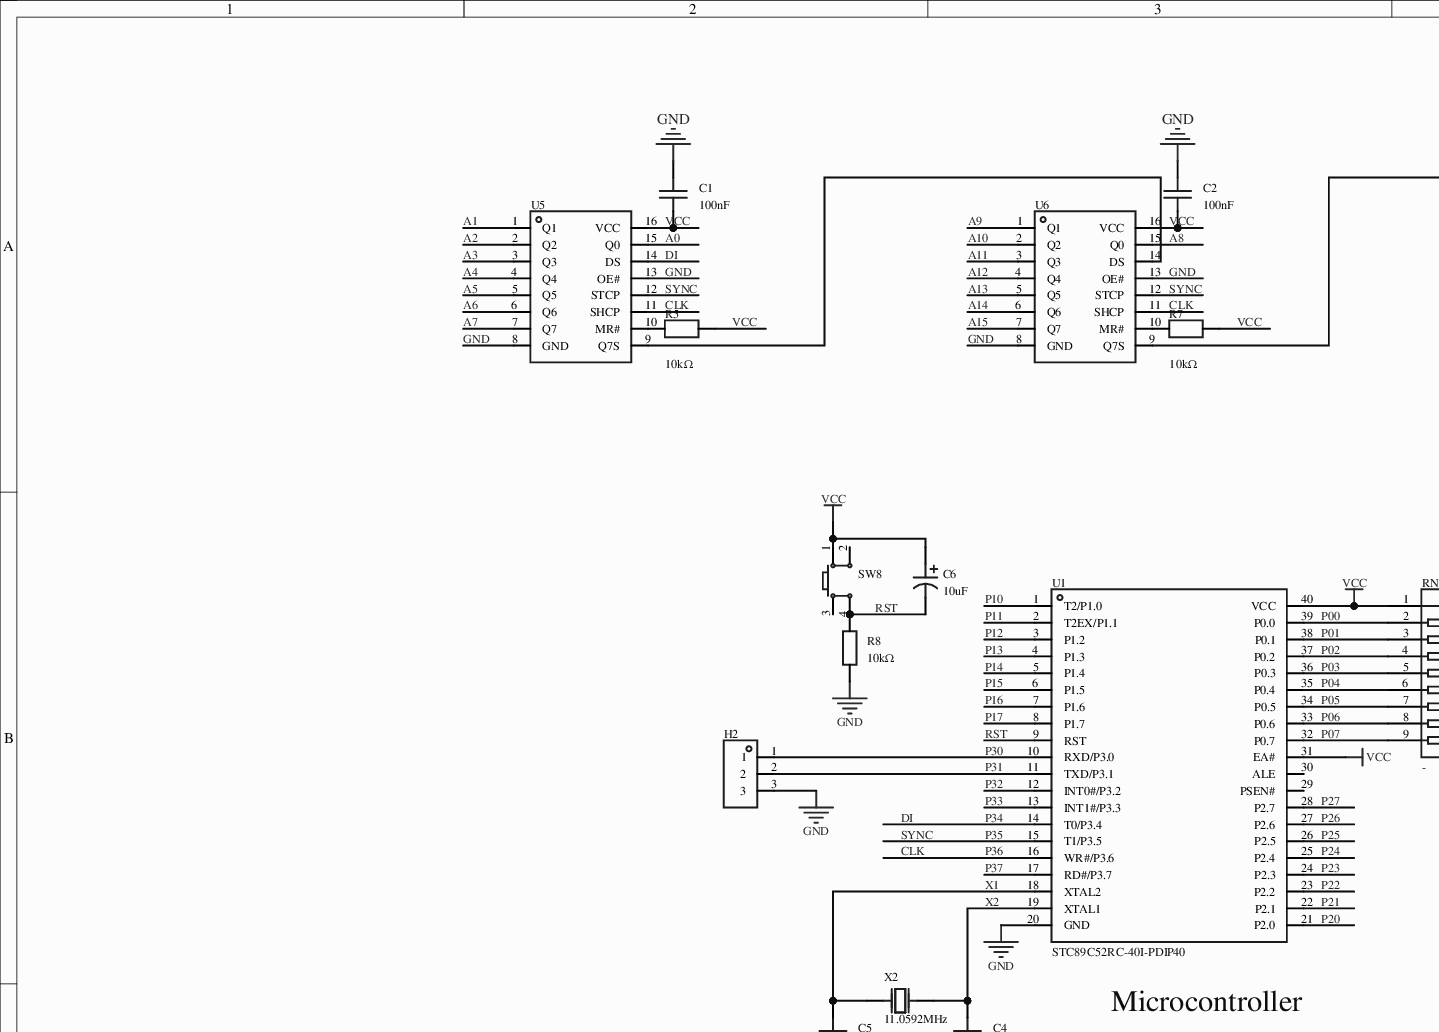
[diagram p0: MISC62490-3.schdoc, top left]
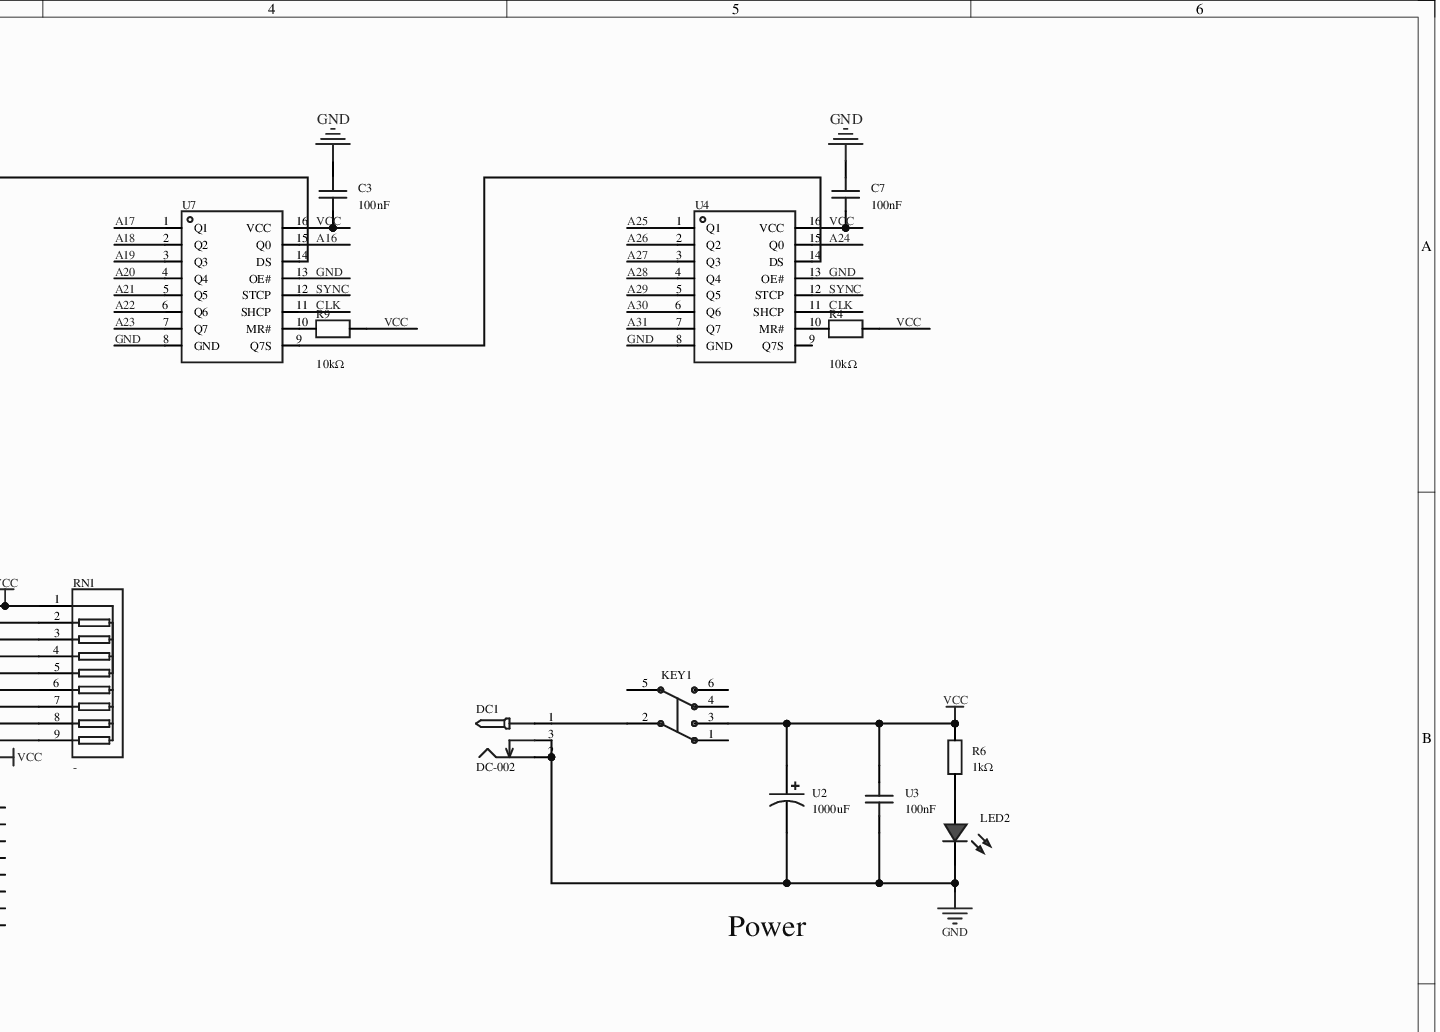
[diagram p1: MISC62490-3.schdoc, top right]
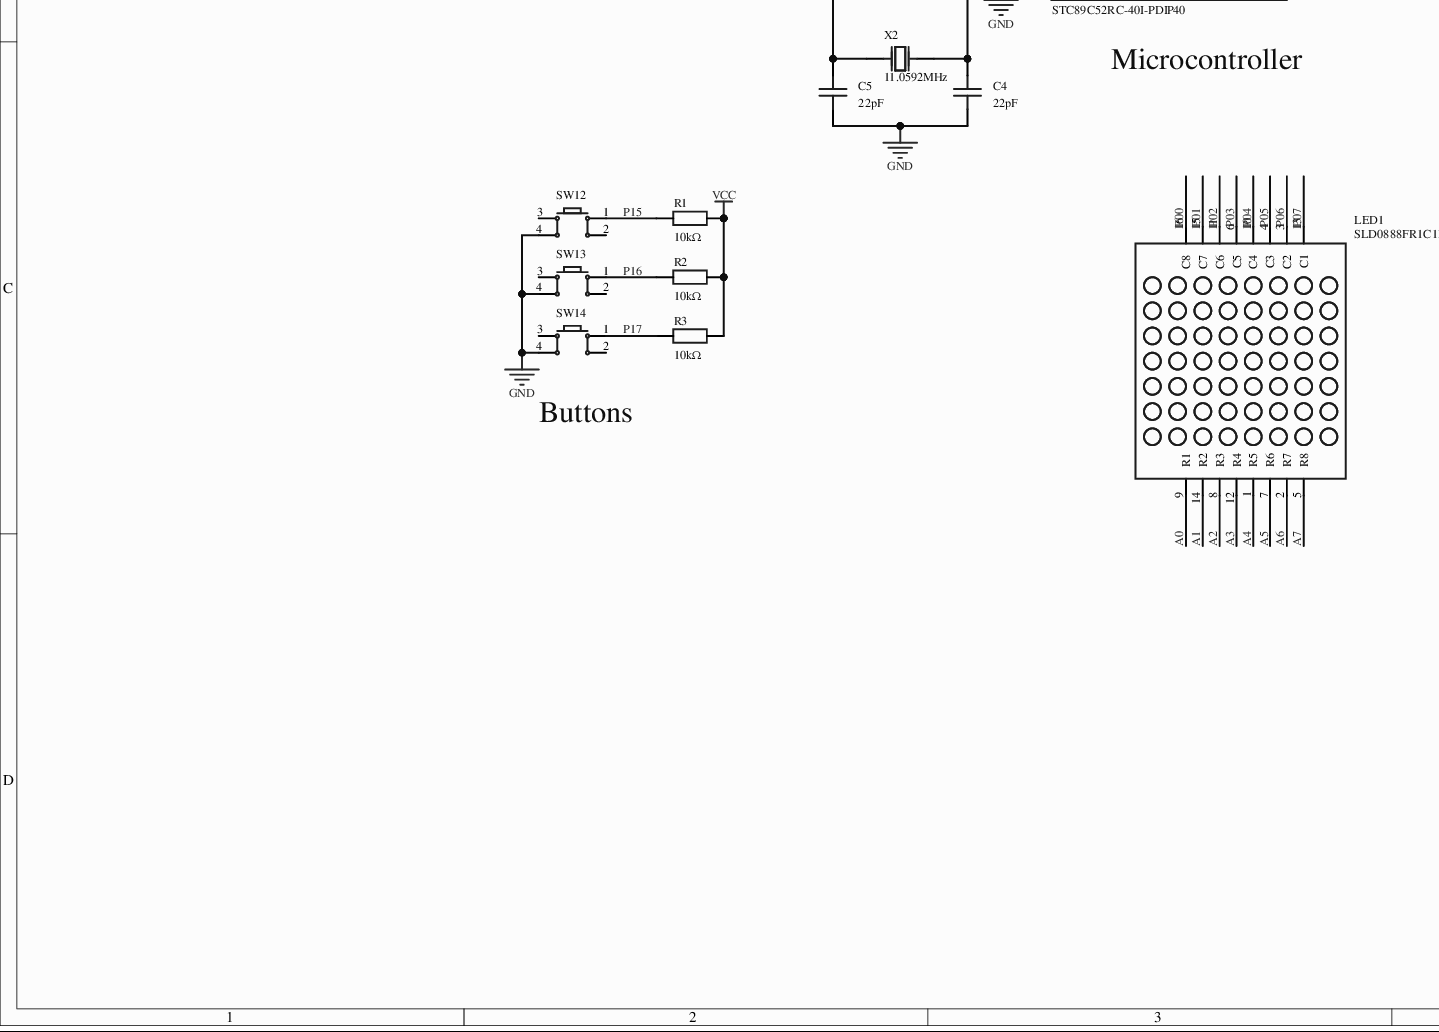
[diagram p2: MISC62490-3.schdoc, bottom left]
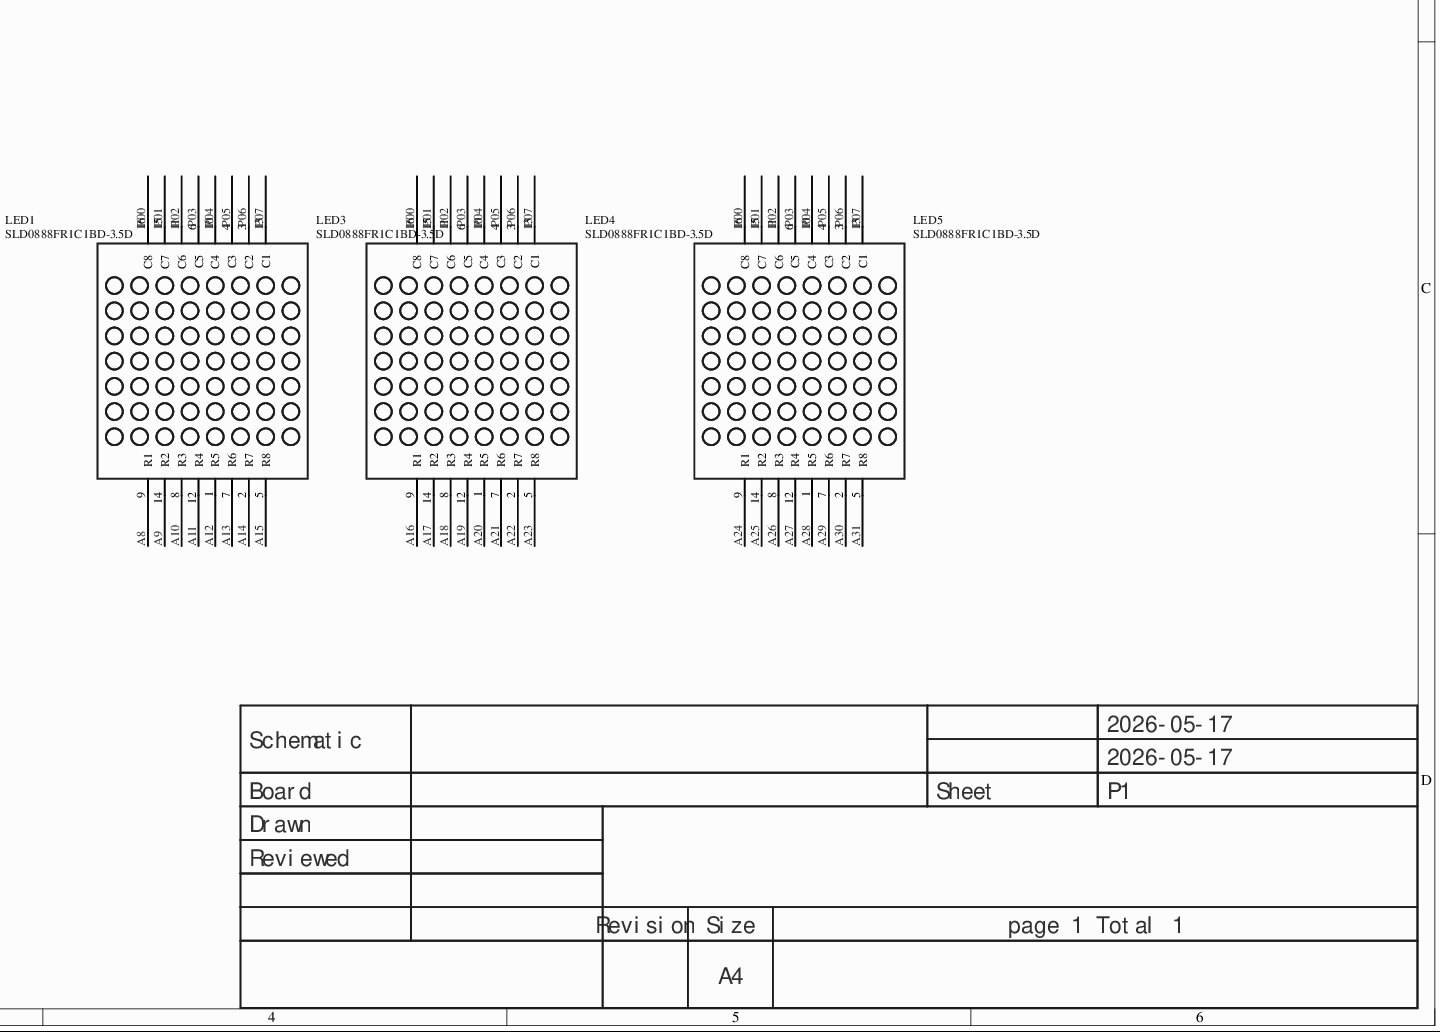
[diagram p3: MISC62490-3.schdoc, bottom right]
# Altium project MISC62490-2.PrjPcb
1 sheet, 37 parts. Net scope: global (net labels, ports and power ports of the same name join across sheets).
Board file: MISC62490.pcbdoc

## Sheet MISC62490-3.schdoc
size 420 x 297 mm; Version: V1.0; @Project Name: MISC62490; @Update Date: 2026-05-17; @Create Date: 2026-05-17; @Board Name: MISC62490; @Create Time: 10:13:01; @Page Count: 1; @Page No: 1; @Schematic Name: MISC62490; @Update Time: 10:13:01; Size: A4

### Parts
C1  100nF  [C0603]
C2  100nF  [C0603]
C3  100nF  [C0603]
C4  22pF  [CAP-TH_L3.8-W2.5-P2.54-D0.50]
C5  22pF  [CAP-TH_L3.8-W2.5-P2.54-D0.50]
C6  10uF  [CAP-TH_BD5.0-P2.00-D0.8-FD-10UF50VC110GL]
C7  100nF  [C0603]
DC1  DC-002  [DC-IN-TH_DC-3510]
H2  (no value)  [HDR-TH_3P-P2.54-V-M]
KEY1  Non-latching switch 8.5×8.5 silent  [SW-TH_6P-L8.5-W8.5-P2.54]  (value not drawn)
LED1  SLD0888FR1C1BD-3.5D  [LED-MAT-TH_SLD0888FR1C1BD-3.5D]
LED2  (no value)  [LED_TH-3mm]
LED3  SLD0888FR1C1BD-3.5D  [LED-MAT-TH_SLD0888FR1C1BD-3.5D]
LED4  SLD0888FR1C1BD-3.5D  [LED-MAT-TH_SLD0888FR1C1BD-3.5D]
LED5  SLD0888FR1C1BD-3.5D  [LED-MAT-TH_SLD0888FR1C1BD-3.5D]
R1  10kΩ  [Res_1/8W]
R2  10kΩ  [Res_1/8W]
R3  10kΩ  [Res_1/8W]
R4  10kΩ  [R0402]
R5  10kΩ  [R0402]
R6  1kΩ  [Res_1/8W]
R7  10kΩ  [R0402]
R8  10kΩ  [Res_1/8W]
R9  10kΩ  [R0402]
RN1  -  [RES-ARRAY-TH_9P-P2.54-D1.0]
SW8  (no value)  [SW-TH_4P-L6.0-W6.0-P4.50-LS6.5]
SW12  (no value)  [SW-TH_4P-L6.0-W6.0-P4.50-LS6.5]
SW13  (no value)  [SW-TH_4P-L6.0-W6.0-P4.50-LS6.5]
SW14  (no value)  [SW-TH_4P-L6.0-W6.0-P4.50-LS6.5]
U1  STC89C52RC-40I-PDIP40  [DIP-40_L52.0-W13.7-P2.54-LS15.2-BL]
U2  1000uF  [CAP-TH_BD12.5-P5.00-D0.6-FD]
U3  100nF  [CAP-TH_L5.0-W2.5-P5.00-D1.0]
U4  74HC595D,118  [SOIC-16_L9.9-W3.9-P1.27-LS6.0-BL]  (value not drawn)
U5  74HC595D,118  [SOIC-16_L9.9-W3.9-P1.27-LS6.0-BL]  (value not drawn)
U6  74HC595D,118  [SOIC-16_L9.9-W3.9-P1.27-LS6.0-BL]  (value not drawn)
U7  74HC595D,118  [SOIC-16_L9.9-W3.9-P1.27-LS6.0-BL]  (value not drawn)
X2  11.0592MHz  [OSC-TH_L11.1-W4.7-P4.88]

### Nets
GND: C1.1 C2.1 C3.1 C4.1 C5.1 C7.1 DC1.2 DC1.3 H2.3 LED2.2(A) R8.1 SW12.4 SW13.4 SW14.4 U1.20(GND) U2.2 U3.2 U4.8(GND) U4.13(OE#) U5.8(GND) U5.13(OE#) U6.8(GND) U6.13(OE#) U7.8(GND) U7.13(OE#)
VCC: C1.2 C2.2 C3.2 C6.1 C7.2 KEY1.3 R1.2 R2.2 R3.2 R4.2 R5.2 R6.2 R7.2 R9.2 RN1.1 SW8.1 U1.31(EA#) U1.40(VCC) U2.1 U3.1 U4.16(VCC) U5.16(VCC) U6.16(VCC) U7.16(VCC)
A0: LED1.9(R1) U5.15(Q0)
A1: LED1.14(R2) U5.1(Q1)
A2: LED1.8(R3) U5.2(Q2)
A3: LED1.12(R4) U5.3(Q3)
A4: LED1.1(R5) U5.4(Q4)
A5: LED1.7(R6) U5.5(Q5)
A6: LED1.2(R7) U5.6(Q6)
A7: LED1.5(R8) U5.7(Q7)
A8: LED3.9(R1) U6.15(Q0)
A9: LED3.14(R2) U6.1(Q1)
A10: LED3.8(R3) U6.2(Q2)
A11: LED3.12(R4) U6.3(Q3)
A12: LED3.1(R5) U6.4(Q4)
A13: LED3.7(R6) U6.5(Q5)
A14: LED3.2(R7) U6.6(Q6)
A15: LED3.5(R8) U6.7(Q7)
A16: LED4.9(R1) U7.15(Q0)
A17: LED4.14(R2) U7.1(Q1)
A18: LED4.8(R3) U7.2(Q2)
A19: LED4.12(R4) U7.3(Q3)
A20: LED4.1(R5) U7.4(Q4)
A21: LED4.7(R6) U7.5(Q5)
A22: LED4.2(R7) U7.6(Q6)
A23: LED4.5(R8) U7.7(Q7)
A24: LED5.9(R1) U4.15(Q0)
A25: LED5.14(R2) U4.1(Q1)
A26: LED5.8(R3) U4.2(Q2)
A27: LED5.12(R4) U4.3(Q3)
A28: LED5.1(R5) U4.4(Q4)
A29: LED5.7(R6) U4.5(Q5)
A30: LED5.2(R7) U4.6(Q6)
A31: LED5.5(R8) U4.7(Q7)
CLK: U1.16(WR#/P3.6) U4.11(SHCP) U5.11(SHCP) U6.11(SHCP) U7.11(SHCP)  [also labelled P36]
DI: U1.14(T0/P3.4) U5.14(DS)  [also labelled P34]
P00: LED1.16(C8) LED3.16(C8) LED4.16(C8) LED5.16(C8) RN1.2 U1.39(P0.0)
P01: LED1.15(C7) LED3.15(C7) LED4.15(C7) LED5.15(C7) RN1.3 U1.38(P0.1)
P02: LED1.11(C6) LED3.11(C6) LED4.11(C6) LED5.11(C6) RN1.4 U1.37(P0.2)
P03: LED1.6(C5) LED3.6(C5) LED4.6(C5) LED5.6(C5) RN1.5 U1.36(P0.3)
P04: LED1.10(C4) LED3.10(C4) LED4.10(C4) LED5.10(C4) RN1.6 U1.35(P0.4)
P05: LED1.4(C3) LED3.4(C3) LED4.4(C3) LED5.4(C3) RN1.7 U1.34(P0.5)
P06: LED1.3(C2) LED3.3(C2) LED4.3(C2) LED5.3(C2) RN1.8 U1.33(P0.6)
P07: LED1.13(C1) LED3.13(C1) LED4.13(C1) LED5.13(C1) RN1.9 U1.32(P0.7)
P10: U1.1(T2/P1.0)
P11: U1.2(T2EX/P1.1)
P12: U1.3(P1.2)
P13: U1.4(P1.3)
P14: U1.5(P1.4)
P15: R1.1 SW12.1 U1.6(P1.5)
P16: R2.1 SW13.1 U1.7(P1.6)
P17: R3.1 SW14.1 U1.8(P1.7)
P20: U1.21(P2.0)
P21: U1.22(P2.1)
P22: U1.23(P2.2)
P23: U1.24(P2.3)
P24: U1.25(P2.4)
P25: U1.26(P2.5)
P26: U1.27(P2.6)
P27: U1.28(P2.7)
P30: H2.1 U1.10(RXD/P3.0)
P31: H2.2 U1.11(TXD/P3.1)
P32: U1.12(INT0#/P3.2)
P33: U1.13(INT1#/P3.3)
P35: U1.15(T1/P3.5) U4.12(STCP) U5.12(STCP) U6.12(STCP) U7.12(STCP)  [also labelled SYNC]
P37: U1.17(RD#/P3.7)
RST: C6.2 R8.2 SW8.4 U1.9(RST)
X1: C5.2 U1.18(XTAL2) X2.1(OSC1)
X2: C4.2 U1.19(XTAL1) X2.2(OSC2)
NetDC1_1: DC1.1 KEY1.2
NetLED2_1: LED2.1(C) R6.1
NetR4_1: R4.1 U4.10(MR#)
NetR5_1: R5.1 U5.10(MR#)
NetR7_1: R7.1 U6.10(MR#)
NetR9_1: R9.1 U7.10(MR#)
NetU4_14: U4.14(DS) U7.9(Q7S)
NetU5_9: U5.9(Q7S) U6.14(DS)
NetU6_9: U6.9(Q7S) U7.14(DS)

Not connected (* = marked no-connect by the designer): KEY1 1 4 5 6; SW8 2 3; SW12 2 3; SW13 2 3; SW14 2 3; U1 29(PSEN#)* 30(ALE)*; U4 9(Q7S)*

### Notes on the sheet
- Power
- (near U1) Microcontroller
- Buttons
- 2026-05-17
- Schematic
- Board
- Sheet
- P1
- Drawn
- Reviewed
- Revision
- Size
- A4
- page 1 Total 1

### Library data of the parts
C1-C3 C7 = FN18X104K500GBG: Capacitance: 100nF; tolerance: ±10%; rated voltage: 50V; temperature coefficient: X7R;; Manufacturer: PSA(信昌电陶); 3D Model: ac125912035d415993ca9572d50418b1; 3D Model Transform: 62.992,31.496,0,0,0,0,0,0,0; AddInBom: yes; ModelName: C0603_L1.6-W0.8-H0.8; Symbol: FN18X104K500GBG; Device: FN18X104K500GBG; Value: 100nF; LCSC Part Name: 100nF ±10% 50V; Supplier Part: C2687355; Manufacturer Part: FN18X104K500GBG; Supplier Footprint: 0603; JLCPCB Part Class: Extended library; Datasheet: example.com/upload/public/pdf/source/20190530/C394159_0C27B7C3BD562F6422EEB4EC92C9B30A.pdf; Supplier: LCSC; Tolerance: ±10%; Voltage Rating: 50V; Temperature Coefficient: X7R; ConvertToPcb: yes; FootprintName: C0603
C4 C5 = C315C300K3G5TA7301: Capacitance: 30pF; tolerance: ±10%; rated voltage: 25V; temperature coefficient: C0G;; Manufacturer: KEMET(基美); 3D Model: 0be8c650c9044d099e9add656cc6dda60819f05c4eef4c71ace90d822a990e87; 3D Model Transform: 149.606,98.8187,0,0,0,0,0,0,-196.85; Pin Spacing: 2.54mm; AddInBom: yes; Symbol: C315C300K3G5TA7301; Device: C315C300K3G5TA7301; LCSC Part Name: 30pF ±10% 25V; Manufacturer Part: C315C300K3G5TA7301; Supplier Footprint: 插件,P=2.54mm; JLCPCB Part Class: Extended Part; Datasheet: example.com/datasheet/C315C300K3G5TA7301/2337370.html; Supplier: LCSC; Value: 22pF; Tolerance: ±10%; Voltage Rating: 25V; Temperature Coefficient: C0G; ConvertToPcb: yes; FootprintName: CAP-TH_L3.8-W2.5-P2.54-D0.50; ModelName: CAP-TH_L3.8-W2.5-P2.54-D0.50
C6 = 10UF50VC110GL: Capacitance: 10uF; tolerance: ±20%; rated voltage: 50V; ripple current: 120mA@100KHz; equivalent series resistance (ESR): 1.6Ω;; Manufacturer: Econd(米朗电子); Pin Spacing: 2mm; Lifetime: 5000hrs@105℃; AddInBom: yes; Symbol: 10UF50VC110GL; Device: 10UF50VC110GL; LCSC Part Name: 10uF ±20% 50V; Supplier Part: C46867109; Manufacturer Part: 10UF50VC110GL; Supplier Footprint: 插件,D5xL11mm; JLCPCB Part Class: Extended Part; Datasheet: example.com/datasheet/10UF50VC110GL/49031974.html; Supplier: LCSC; Value: 10uF; Tolerance: ±20%; Voltage Rating: 50V; Ripple Current: 120mA@100KHz; Equivalent Series Resistance(ESR): 1.6Ω; Diameter: 5mm; Height - Seated (Max): 11mm; Operating Temperature: -40℃~+105℃; ConvertToPcb: yes; FootprintName: CAP-TH_BD5.0-P2.00-D0.8-FD-10UF50VC110GL
DC1 = DC-002: 3D Model: 28059cb5f325411c86e5e1af88d5b1310819f05c4eef4c71ace90d822a990e87; 3D Model Transform: 450.787,208.661,0,180,0,0,113.189,-47.244,-125.984; AddInBom: yes; Symbol: DC-002; Device: DC-002; LCSC Part Name: DC-002 铁脚 内铁芯1.0mm; Supplier Part: C12568; Manufacturer Part: DC-002; Supplier Footprint: 插件; JLCPCB Part Class: Extended Part; Supplier: LCSC; ConvertToPcb: yes; FootprintName: DC-IN-TH_DC-3510; ModelName: DC-IN-TH_DC-3510
H2 = HDR-M_2.54_1x3P: 3D Model: bb473b6d38ff42a99216a4fcdbdcc4cb0819f05c4eef4c71ace90d822a990e87; 3D Model Transform: 300.03877,100,0,0,0,0,0,0,-118.11; AddInBom: yes; ModelName: HDR-TH_3P-P2.54-M-LI-1X3P; Symbol: HDR-M_2.54_1x3P; Device: HDR-M_2.54_1x3P; Supplier Part: C2937625; Supplier Footprint: 插件; ConvertToPcb: yes; FootprintName: HDR-TH_3P-P2.54-V-M
KEY1 = 无自锁开关 8.5×8.5 无声: 6 pins, 8.5×8.5; Symbol: No self-locking switch 8.5×8.5 silent; 3D Model: 4c72b3966b92446eb355e1bd0fb4f8800819f05c4eef4c71ace90d822a990e87; 3D Model Transform: 342.519,334.645,0,180,0,0,0,0,-137.795; AddInBom: yes; Device: Non-latching switch 8.5×8.5 silent; LCSC Part Name: 无自锁开关 8.5×8.5  无声; Supplier Part: C26228; Manufacturer Part: 无自锁开关 8.5×8.5 无声; Supplier Footprint: 插件; JLCPCB Part Class: Extended Part; Supplier: LCSC; ConvertToPcb: yes; FootprintName: SW-TH_6P-L8.5-W8.5-P2.54; ModelName: SW-TH_6P-L8.5-W8.5-P2.54
LED1 LED3-LED5 = SLD0888FR1C1BD-3.5D: Digits: 8x8; luminous color: red; polarity: common cathode;; Manufacturer: SUNLIGHT(光华); AddInBom: yes; ModelId: 95faf80081c74ca5b80a70d04b8b65640819f05c4eef4c71ace90d822a990e87; ModelTransform: 787.4,787.7937,0,0,0,0,0,0,-137.795; Symbol: SLD0888FR1C1BD-3.5D; Device: SLD0888FR1C1BD-3.5D; LCSC Part Name: 点阵; SupplierPart: C42378520; ManufacturerPart: SLD0888FR1C1BD-3.5D; Supplier Footprint: 插件; Datasheet: example.com/datasheet/SLD0888FR1C1BD-3.5D/44281439.html; Supplier: LCSC; ConvertToPcb: yes; FootprintName: LED-MAT-TH_SLD0888FR1C1BD-3.5D; ModelName: LED-MAT-TH_SLD0888FR1C1BD-3.5D; Number of Digits: 8x8; Illumination Color: Red; Polarity: Common cathode
LED2 = LED_TH-R_3mm: 3D Model: a497c992633541038a38947cdc58012f0819f05c4eef4c71ace90d822a990e87; 3D Model Transform: 141.274,153.327,0,0,0,0,-5.984,0,-137.795; ConvertToPcb: yes; ModelName: LED-TH-3mm_R; Symbol: LED_TH-R; Device: LED_TH-R_3mm; Supplier Footprint: 插件; AddInBom: yes; FootprintName: LED_TH-3mm
R1-R3 R6 R8 = Res_AXIAL-1/8W: Symbol: Resistor; 3D Model: b2b5ae7ae4c642178fe0039925c86a3f0819f05c4eef4c71ace90d822a990e87; 3D Model Transform: 282.86,66.88,253.09,0,0,0,0,0,-191; ConvertToPcb: yes; ModelName: RES-TH_BD1.8-L3.2-P7.20-D0.4; Device: Res_AXIAL-1/8W; Supplier Footprint: 轴向引线; AddInBom: yes; FootprintName: Res_1/8W
  R1-R3 R8: Value: 10kΩ
  R6: Value: 1kΩ
R4 R5 R7 R9 = RCA0210KJLF: Resistance: 10kΩ; tolerance: ±5%; power: 62.5mW;; Manufacturer: HKR(香港电阻); 3D Model: 98c88bc2b9094f218f3a3e30a7012738; 3D Model Transform: 39.37,19.685,0,0,0,0,0,0,0; AddInBom: yes; ModelName: R0402_L1.0-W0.5-H0.4; Symbol: RCA0210KJLF; Device: RCA0210KJLF; Value: 10kΩ; LCSC Part Name: 10kΩ ±5% 62.5mW; Supplier Part: C22356213; Manufacturer Part: RCA0210KJLF; Supplier Footprint: 0402; JLCPCB Part Class: Extended library; Datasheet: example.com/upload/public/pdf/source/20240312/EB29F8B3E9AD4CE07E65E9956C47F4F5.pdf; Supplier: LCSC; Tolerance: ±5%; Power(Watts): 62.5mW; ConvertToPcb: yes; FootprintName: R0402
RN1 = 排阻 10 K 5%: Number of resistors: -; resistance: -; power per element: -;; Symbol: 10 K 5%; Device: Resistor array 10 K 5%; AddInBom: yes; ModelId: d106c67f29e14d8080ba548247a719a10819f05c4eef4c71ace90d822a990e87; ModelName: SIP-9_L22.8-W3.0-H8.5-P2.54; ModelTransform: 918.1084,118.11,0,0,0,0,0,0,-137.795; LCSC Part Name: 10KΩ (103) ±5%; SupplierPart: C26615; ManufacturerPart: 排阻 10 K 5%; Supplier Footprint: 插件; JLCPCB Part Class: Extended Part; Supplier: LCSC; ConvertToPcb: yes; FootprintName: RES-ARRAY-TH_9P-P2.54-D1.0; Number of Resistors: -; Value: -; Power(Watts): -; Number of Pins: -
SW8 SW12-SW14 = Key_TH_6x6x6: Contact current: 50mA; rated voltage (DC): 12V; insulation resistance: 100MΩ; circuit structure: SPST; mounting: through-hole; button shape: round button; button/cap color: black; actuation force: 260gf@±30gf; operating temperature: -25℃~+70℃; pin style: PC pin; switch length: 6mm; switch width: 6mm; switch height: 6mm; with bracket: no;; Symbol: Tactile switch; 3D Model: 20eee248bc684ccd8cbdbb1d0d91ec6f0819f05c4eef4c71ace90d822a990e87; 3D Model Transform: 236.22,323.03,0,90,0,0,0,0,-137.795; AddInBom: yes; ModelName: SW-TH_4P-L6.0-W6.0-H5.0-LS6.5-P4.50; Device: Key_TH_6x6x6; Supplier Footprint: 插件; ConvertToPcb: yes; FootprintName: SW-TH_4P-L6.0-W6.0-P4.50-LS6.5
U1 = STC89C52RC-40I-PDIP40: CPU core: 51 family; max CPU frequency: -;; Manufacturer: STC; AddInBom: yes; ModelId: 16d4686a009b4ddca948f91eddb57b140819f05c4eef4c71ace90d822a990e87; ModelName: DIP-40_L52.3-W13.8-H4.0-LS15.24-P2.54; ModelTransform: 2059.051,615.743,0,0,0,0,0,0,-118.11; Program Storage Size: 8KB; Program Memory Type: FLASH; Voltage - Supply: 3.3V~5.5V; Symbol: STC89C52RC-40I; Device: STC89C52RC-40I-PDIP40; LCSC Part Name: 单片机原理及应用; SupplierPart: C14022; ManufacturerPart: STC89C52RC-40I-PDIP40; Supplier Footprint: DIP-40; JLCPCB Part Class: Extended Part; Datasheet: example.com/datasheet/STC89C52RC-40I-PDIP40/14679.html; Supplier: LCSC; ConvertToPcb: yes; FootprintName: DIP-40_L52.0-W13.7-P2.54-LS15.2-BL; CPU Core: 51 family; CPU Maximum Speed: -; RAM Size: -; EEPROM: -; Number of I/O: -; ADC (Bit): -; DAC (Bit): -
U2 = 35YK1000M12.5X20: Capacitance: 1000uF; tolerance: ±20%; rated voltage: 35V; ripple current: 1.18A@120Hz; equivalent series resistance (ESR): -;; Manufacturer: Rubycon(红宝石); Symbol: 35YK1000M12.5X20_C1596673; AddInBom: yes; ModelId: 968d8ff988964aab8919b46a6a737be20819f05c4eef4c71ace90d822a990e87; ModelName: CAP-TH_D12.5-H20.0-P5.00; ModelTransform: 492.5187,492.11201,0,0,0,0,0,0,-137.795; Pin Spacing: 5mm; Lifetime: 2000hrs@85℃; Device: 35YK1000M12.5X20; LCSC Part Name: 1000uF ±20% 35V; SupplierPart: C1596673; ManufacturerPart: 35YK1000M12.5X20; Supplier Footprint: 插件,D12.5xL20mm; JLCPCB Part Class: Extended Part; Datasheet: example.com/upload/public/pdf/source/20210510/C1596673_C6EAD3AB6CF7008EAB8FD89AA98F8A2E.pdf; Supplier: LCSC; ConvertToPcb: yes; FootprintName: CAP-TH_BD12.5-P5.00-D0.6-FD; Value: 1000uF; Tolerance: ±20%; Voltage Rating: 35V; Ripple Current: 1.18A@120Hz; Equivalent Series Resistance(ESR): -; Diameter: 12.5mm; Height - Seated (Max): 20mm; Operating Temperature: -25℃~+85℃
U3 = 100nF: Symbol: 100NF_C9900015256; AddInBom: yes; ModelId: 08e3d7481fc7486bb1b263873f51e1e10819f05c4eef4c71ace90d822a990e87; ModelName: CAP-TH_BD5.0-W2.5-P5.08; ModelTransform: 224.652,98.425,0,0,0,0,-0.005,0,-137.795; Device: 100nF; LCSC Part Name: 100nF; SupplierPart: C9900015256; ManufacturerPart: 100nF; Supplier Footprint: CAP-TH_L5.0-W2.5-P5.00-D1.0; JLCPCB Part Class: Extended Part; Supplier: LCSC; ConvertToPcb: yes; FootprintName: CAP-TH_L5.0-W2.5-P5.00-D1.0
U4-U7 = 74HC595D,118: Function: serial-to-serial or parallel; supply voltage: 2V~6V; number of elements: 1; bits per element: 8;; Manufacturer: Nexperia(安世); 3D Model: c21ec766ec2643efb3352f8441994f4e; 3D Model Transform: 389.763,236.454,0,0,0,0,0,0,0; Number of Elements: 1; Number of Bits per Element: 8; Output Type: Three-state; AddInBom: yes; ModelName: SOIC-16_L9.9-W3.9-H1.8-LS6.0-P1.27; Symbol: 74HC595D,118; Device: 74HC595D,118; LCSC Part Name: 三态输出 串行至串行或并行移位寄存器; Supplier Part: C5947; Manufacturer Part: 74HC595D,118; Supplier Footprint: SOIC-16; JLCPCB Part Class: Basic library; Datasheet: example.com/upload/public/pdf/source/20240724/C3A3241CA190230F407C83CEC4244600.pdf; Supplier: LCSC; Function: Serial-to-serial or parallel; Supply Voltage: 2V~6V; Series: 74HC; Operating Temperature: -40℃~+125℃; ConvertToPcb: yes; FootprintName: SOIC-16_L9.9-W3.9-P1.27-LS6.0-BL
X2 = 9AC11059302060C3: Crystal type: through-hole crystal; frequency: 11.0592MHz; room-temperature tolerance: ±20ppm; load capacitance: 30pF;; Manufacturer: JGHC(晶光华); 3D Model: f2ed30de83344a4b83b1c4b1b9fe18560819f05c4eef4c71ace90d822a990e87; 3D Model Transform: 436.37503,185.039,0,0,0,0,0,0,-137.795; Equivalent Series Resistance(ESR): 60Ω; AddInBom: yes; Symbol: 9AC11059302060C3; Device: 9AC11059302060C3; LCSC Part Name: 11.0592MHz ±20ppm 30pF; Supplier Part: C2715911; Manufacturer Part: 9AC11059302060C3; Supplier Footprint: HC-49S; JLCPCB Part Class: Extended Part; Datasheet: example.com/datasheet/9AC11059302060C3/2832137.html; Supplier: LCSC; Type: Through-hole crystal; Value: 11.0592MHz; Normal temperature Frequency Tolerance: ±20ppm; Load Capacitance: 30pF; Operating Temperature: -40℃~+85℃; ConvertToPcb: yes; FootprintName: OSC-TH_L11.1-W4.7-P4.88; ModelName: OSC-TH_L11.1-W4.7-P4.88